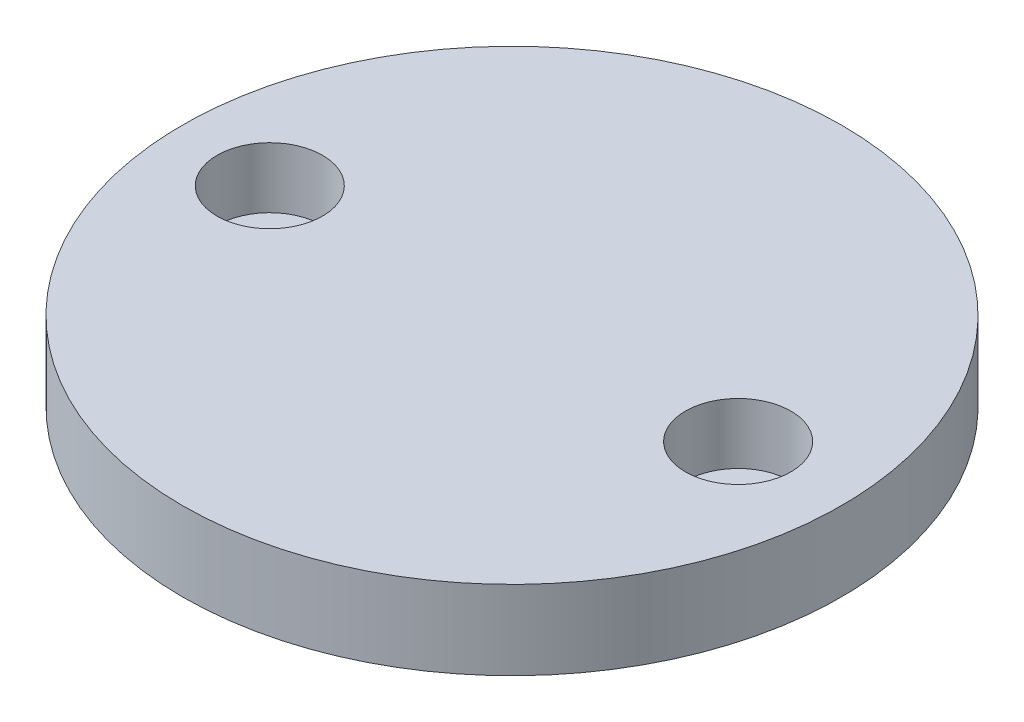
SolidWorks part; units mm, degrees
ref_plane "Front Plane" through (0, 0, 0) normal (0, 0, 1) x (1, 0, 0)
ref_plane "Top Plane" through (0, 0, 0) normal (0, 1, 0) x (1, 0, 0)
ref_plane "Right Plane" through (0, 0, 0) normal (1, 0, 0) x (0, 0, -1)
sketch "Sketch1" plane through (0, 0, 0) normal (0, 1, 0) x (1, 0, 0)
  circle A0 centre (0, 0) radius 25
  dimension "D1" = 50
extrude "Boss-Extrude1" add sketch "Sketch1" along normal blind 6
sketch "Sketch2" plane through (0, 6, 0) normal (0, 1, 0) x (1, 0, 0)
  point P0 (16.8647, 0.2895)
  point P1 (-17.7033, -0.6722)
hole_wizard "Hole size based on socket head cap screw type 1" positions "3DSketch1" profile "Sketch3" counterbore size "M4" standard "GB"
sketch3d "3DSketch1"
  point P0 (16.8647, 6, -0.2895)
  point P3 (-17.7033, 6, 0.6722)
sketch "Sketch3" plane through (16.8647, 6, -0.2895) normal (1, 0, 0) x (0, 0, 1)
  line L0 (0, 0) -> (0, 11.4519)
  line L1 (0, 11.4519) -> (2.25, 10.1)
  line L2 (2.25, 10.1) -> (2.25, 4.6)
  line L3 (2.25, 4.6) -> (4, 4.6)
  line L4 (4, 4.6) -> (4, 0)
  line L5 (4, 0) -> (0, 0)
  line L10 (0, 11.4519) -> (-2.25, 10.1) construction
  line L11 (0, -6.35) -> (0, 107.95) construction
  dimension "孔直径" = 4.5
  dimension "孔深度" = 10.1
  dimension "柱形沉头孔直径" = 8
  dimension "柱形沉头孔深度" = 4.6
  dimension "导头角度" = 118
